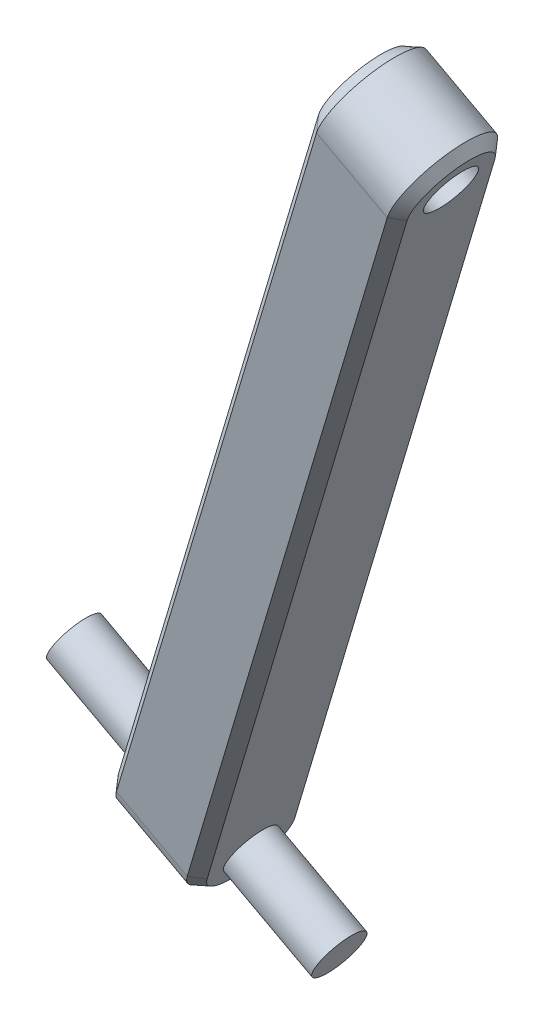
SolidWorks part; units mm, degrees
ref_plane "Front Plane" through (0, 0, 0) normal (0, 0, 1) x (1, 0, 0)
ref_plane "Top Plane" through (0, 0, 0) normal (0, 1, 0) x (1, 0, 0)
ref_plane "Right Plane" through (0, 0, 0) normal (1, 0, 0) x (0, 0, -1)
ref_plane "Plane4" through (14.0293, -7.5365, 0) normal (0.8809, -0.4732, 0) x (0.4732, 0.8809, 0)
sketch "Sketch1" plane through (14.0293, -7.5365, 0) normal (0.8809, -0.4732, 0) x (0.4732, 0.8809, 0)
  line L0 (-90.3906, -267.7386) -> (-32.9195, -250.5028)
  line L1 (-34.3559, -245.7136) -> (-91.827, -262.9493)
  arc A0 (-91.827, -262.9493) -> (-90.3906, -267.7386) centre (-91.1088, -265.344) ccw
  arc A1 (-32.9195, -250.5028) -> (-34.3559, -245.7136) centre (-33.6377, -248.1082) ccw
extrude "Boss-Extrude1" add sketch "Sketch1" against normal blind 5
ref_plane "Plane5" through (0, 0, -265.344) normal (0, 0, 1) x (1, 0, 0)
sketch "Sketch2" plane through (0, 0, -265.344) normal (0, 0, 1) x (1, 0, 0)
  line L0 (-37.3045, -81.964) -> (-37.896, -83.0651)
  line L1 (-37.896, -83.0651) -> (-33.4913, -85.4313)
  line L2 (-33.4913, -85.4313) -> (-32.8998, -84.3302)
  line L3 (-32.8998, -84.3302) -> (-37.3045, -81.964)
  line L4 (-36.9096, -83.5951) -> (-34.4778, -84.9014) construction
revolve "Revolve1" add sketch "Sketch2" angle 360 about L4
sketch "Sketch3" plane through (0, 0, -265.344) normal (0, 0, 1) x (1, 0, 0)
  line L0 (-28.4951, -86.6963) -> (-29.0866, -87.7975)
  line L1 (-29.0866, -87.7975) -> (-24.682, -90.1637)
  line L2 (-24.682, -90.1637) -> (-24.0904, -89.0625)
  line L3 (-24.0904, -89.0625) -> (-28.4951, -86.6963)
  line L4 (-28.1002, -88.3274) -> (-25.6684, -89.6338) construction
revolve "Revolve2" add sketch "Sketch3" angle 360 about L4
hole_wizard "Ø2.5 (2.5) Diameter Hole1" positions "Sketch5" profile "Sketch4" hole size "Ø2.5" standard "ANSI Metric"
sketch "Sketch5" plane through (9.6247, -5.1703, 0) normal (-0.8809, 0.4732, 0) x (0, 0, 1)
  point P0 (-248.1082, -33.6377)
sketch "Sketch4" plane through (-6.2939, -34.803, -248.1082) normal (0, 0, 1) x (-0.4732, -0.8809, 0)
  line L0 (0, 0) -> (0, 31.6423)
  line L1 (0, 31.6423) -> (1.25, 31.6423)
  line L2 (1.25, 31.6423) -> (1.25, 0)
  line L5 (1.25, 0) -> (0, 0)
  line L11 (0, -6.35) -> (0, 107.95) construction
  dimension "通孔孔直径" = 2.5
  dimension "通孔孔深度" = 31.6423
chamfer "Chamfer1" distance 0.5 angle 45 8 edges at (-0.756, -35.0597, -247.39) (-15.1481, -61.8507, -259.1207) (-15.8278, -63.116, -254.3314) (-30.2199, -89.907, -266.0621) (-19.5528, -59.4845, -259.1207) (-34.6245, -87.5408, -266.0621) (-5.1607, -32.6935, -247.39) (-20.2325, -60.7498, -254.3314)
